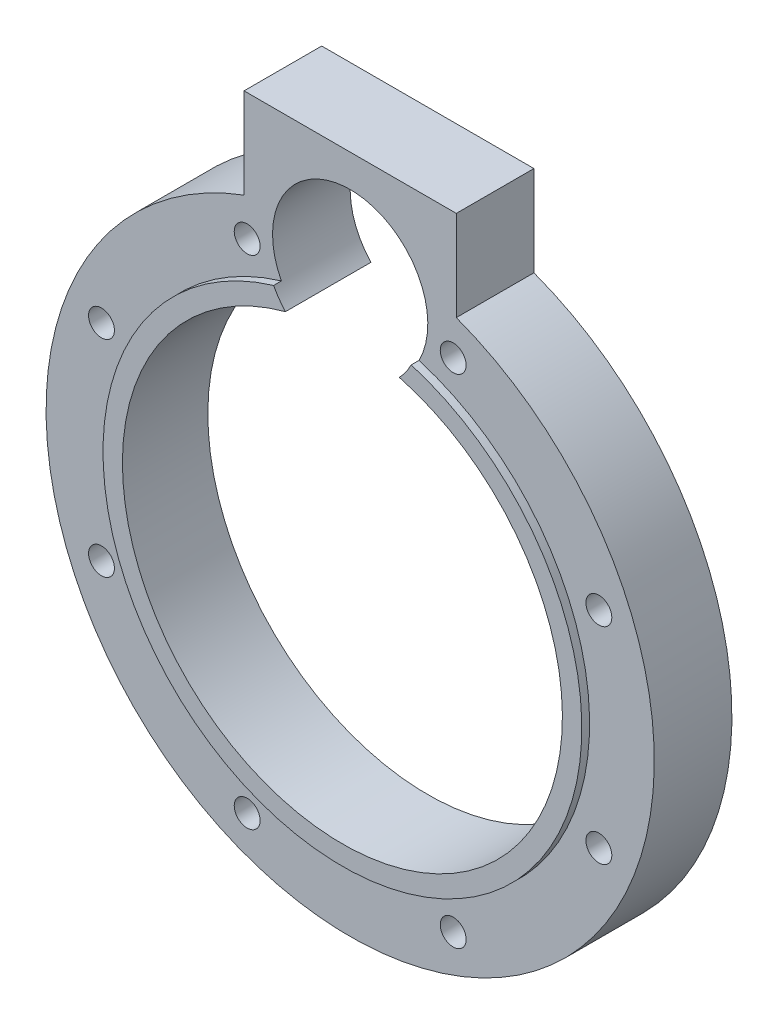
from build123d import *

# Parameters (mm, degrees)
SKETCH_1_R          = 117.5
SKETCH_1_R_2        = 85
EXTRUDE_1_DEPTH     = 30
SKETCH_3_W          = 82
SKETCH_3_H          = 60
EXTRUDE_5_DEPTH     = 30
HOLE_WIZARD_M8_1_D  = 10
SKETCH_9_R          = 92.5
SKETCH_9_R_2        = 85
EXTRUDE_7_DEPTH     = 3
SKETCH_8_R          = 30
CUT_EXTRUDE_1_DEPTH = 190.526383388


with BuildPart() as part:
    # 草图1 → 凸台-拉伸1 (new body)
    with BuildSketch(Plane.XY):
        Circle(SKETCH_1_R)
        Circle(SKETCH_1_R_2, mode=Mode.SUBTRACT)
    extrude(amount=EXTRUDE_1_DEPTH)

    # 草图3 → 凸台-拉伸5 (add, through all)
    with BuildSketch(Plane.XY.offset(30)):
        with Locations((0, 115)):
            Rectangle(SKETCH_3_W, SKETCH_3_H)
    extrude(amount=-EXTRUDE_5_DEPTH)

    # M8 间隙孔1 (through all)
    with Locations(Plane(origin=(0, 0, 0), x_dir=(-1, 0, 0), z_dir=(0, 0, -1))):
        with Locations((-39.799076966, 96.083471381), (39.799076966, 96.083471381), (96.083471381, 39.799076966), (96.083471381, -39.799076966), (39.799076966, -96.083471381), (-39.799076966, -96.083471381), (-96.083471381, -39.799076966), (-96.083471381, 39.799076966)):
            Hole(HOLE_WIZARD_M8_1_D / 2)

    # 草图9 → 凸台-拉伸7 (add)
    with BuildSketch(Plane.XY.offset(30)):
        Circle(SKETCH_9_R)
        Circle(SKETCH_9_R_2, mode=Mode.SUBTRACT)
    extrude(amount=EXTRUDE_7_DEPTH)

    # 草图8 → 切除-拉伸1 (cut, through all)
    with BuildSketch(Plane(origin=(0, 0, 0), x_dir=(-1, 0, 0), z_dir=(0, 0, -1))):
        with Locations((0, 102.5)):
            Circle(SKETCH_8_R)
    extrude(amount=-CUT_EXTRUDE_1_DEPTH, mode=Mode.SUBTRACT)


solid = part.part
